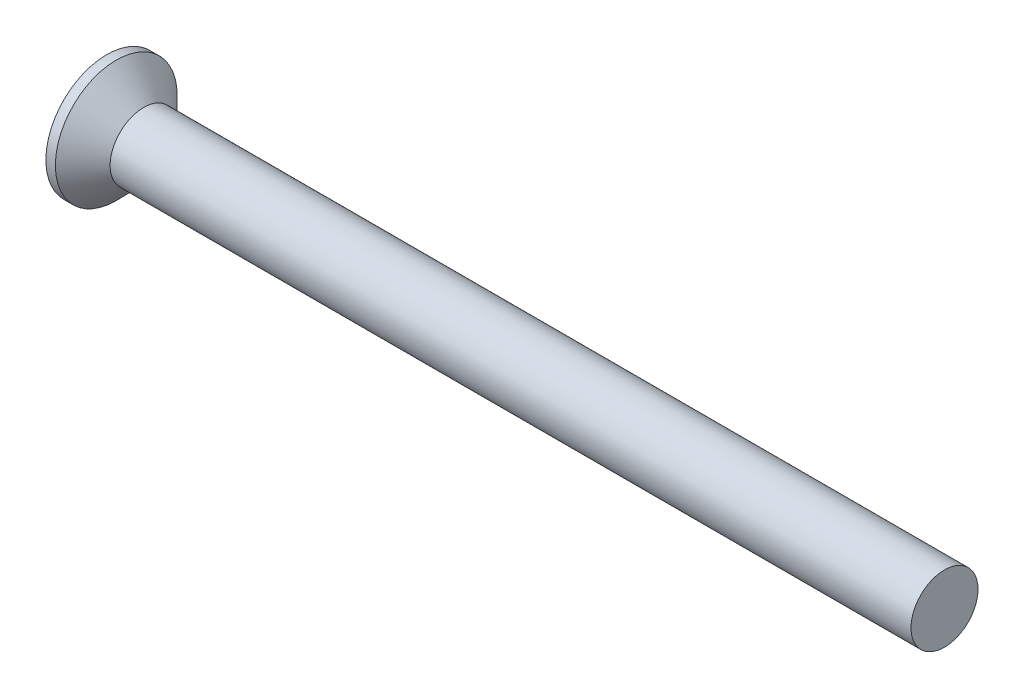
from build123d import *

# Parameters (mm, degrees)
CROSSRECESS_DEPTH = 1.65
DRAFT9_ANGLE      = 30
FILLET5_R         = 0.3
SKETCH10_W        = 1
SKETCH10_H        = 3


with BuildPart() as part:
    # Sketch1 → Base (revolve)
    with BuildSketch(Plane.XY, mode=Mode.PRIVATE) as base_sk:
        Polygon((75, 3), (5.3, 3), (3.3, 3), (0.85, 5.45), (0, 5.45), (0, 0), (75, 0), align=None)
    revolve(base_sk.sketch.rotate(Axis((4.515812911, 0, 0), (-1, 0, 0)), 90), axis=Axis((4.515812911, 0, 0), (-1, 0, 0)))

    # Sketch6 → CrossRecess (cut)
    with BuildSketch(Plane(origin=(0, 0, 0), x_dir=(0, 0, -1), z_dir=(1, 0, 0))):
        Polygon((0.68, 0.68), (0.68, 3.4), (-0.68, 3.4), (-0.68, 0.68), (-3.4, 0.68), (-3.4, -0.68), (-0.68, -0.68), (-0.68, -3.4), (0.68, -3.4), (0.68, -0.68), (3.4, -0.68), (3.4, 0.68), align=None)
    extrude(amount=CROSSRECESS_DEPTH, mode=Mode.SUBTRACT)

    # Draft9
    draft9_faces = [part.faces().sort_by_distance(p)[0] for p in [
        (0.825, -3.4, 0),
        (0.825, 0, 3.4),
        (0.825, 0, -3.4),
        (0.825, 3.4, 0),
    ]]
    draft(draft9_faces, Plane(origin=(0, 5.45, 0), x_dir=(0, 0, -1), z_dir=(-1, 0, 0)), DRAFT9_ANGLE)

    # Fillet5
    fillet5_edges = [part.edges().sort_by_distance(p)[0] for p in [
        (0.825, 0.68, 0.68),
        (0.825, -0.68, 0.68),
        (0.825, -0.68, -0.68),
        (0.825, 0.68, -0.68),
    ]]
    fillet(fillet5_edges, radius=FILLET5_R)

    # Sketch10 → Revolve2 (revolve)
    with BuildSketch(Plane.XY):
        with Locations((3.8, 1.5)):
            Rectangle(SKETCH10_W, SKETCH10_H)
    revolve(axis=Axis((62.228915663, 0, 0), (-1, 0, 0)))


solid = part.part
